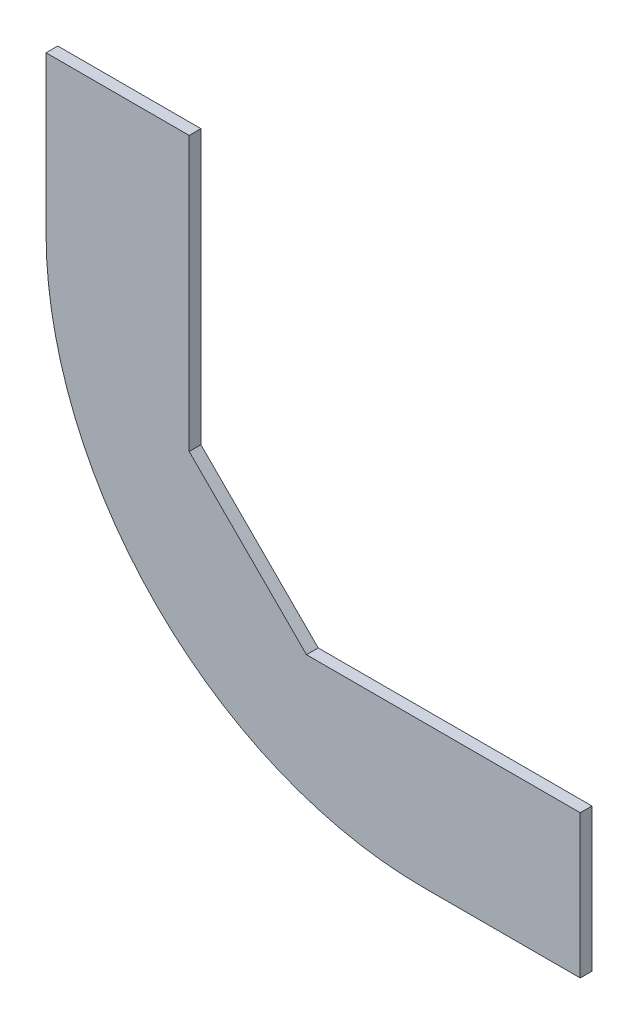
from build123d import *

# Parameters (mm, degrees)
EXTRUDE_1_DEPTH = 1.5


with BuildPart() as part:
    # 草图1 → 凸台-拉伸1 (new body)
    with BuildSketch(Plane.XY):
        with BuildLine():
            Line((28.659646302, 45.489008558), (28.659646302, 25.489008558))
            ThreePointArc((28.659646302, 25.489008558), (42.806388771, -8.664248973), (76.959646302, -22.810991442))
            Line((76.959646302, -22.810991442), (96.959646302, -22.810991442))
            Line((96.959646302, -22.810991442), (96.959646302, -4.510991442))
            Line((96.959646302, -4.510991442), (61.959646302, -4.510991442))
            Line((61.959646302, -4.510991442), (46.959646302, 10.489008558))
            Line((46.959646302, 10.489008558), (46.959646302, 45.489008558))
            Line((46.959646302, 45.489008558), (28.659646302, 45.489008558))
        make_face()
    extrude(amount=EXTRUDE_1_DEPTH)


solid = part.part
